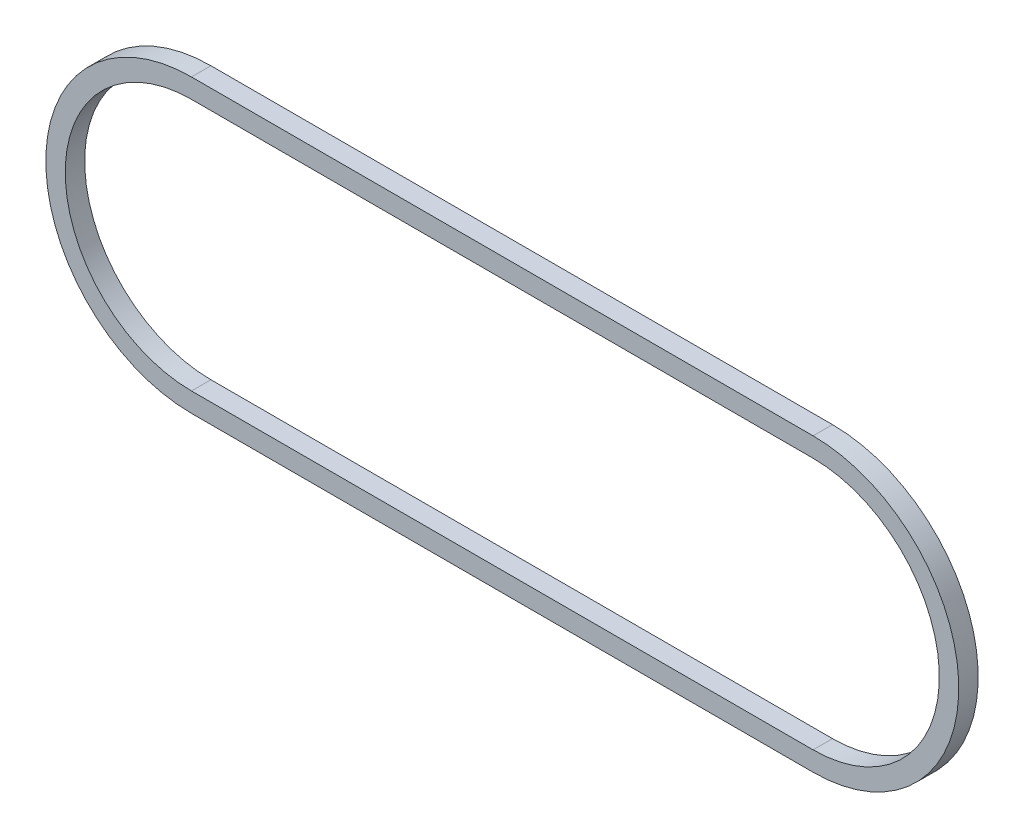
from build123d import *

# Parameters (mm, degrees)
EXTRUDE_1_DEPTH = 10


with BuildPart() as part:
    # 草图1 → 凸台-拉伸1 (new body)
    with BuildSketch(Plane.XY):
        with BuildLine():
            Line((0, 75), (320, 75))
            ThreePointArc((320, 75), (395, 0), (320, -75))
            Line((320, -75), (0, -75))
            ThreePointArc((0, -75), (-75, 0), (0, 75))
        make_face()
        with BuildLine():
            Line((0, 65), (320, 65))
            ThreePointArc((320, 65), (385, 0), (320, -65))
            Line((320, -65), (0, -65))
            ThreePointArc((0, -65), (-65, 0), (0, 65))
        make_face(mode=Mode.SUBTRACT)
    extrude(amount=EXTRUDE_1_DEPTH)


solid = part.part
